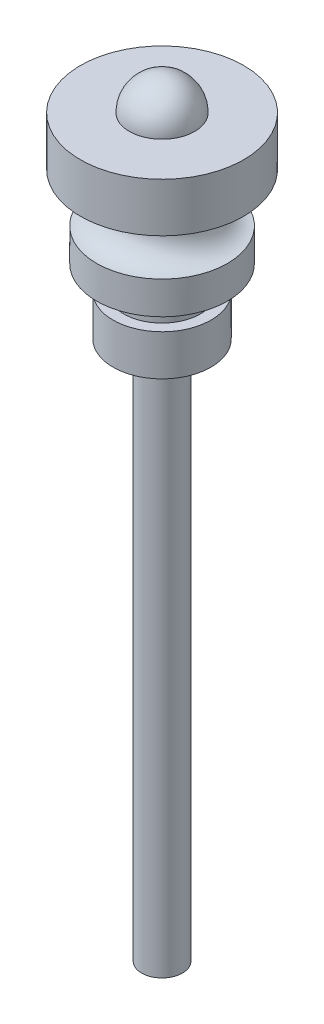
from build123d import *


with BuildPart() as part:
    # Sketch1 → Revolve1 (revolve)
    with BuildSketch(Plane.XY, mode=Mode.PRIVATE) as revolve1_sk:
        Polygon((0, 0), (10, 0), (10, -6), (8, -6), (8, -16), (4.7, -16), (4.7, -19), (6, -19), (6, -24), (2.5, -24), (2.5, -90), (0, -90), align=None)
    revolve(revolve1_sk.sketch.rotate(Axis((0, 0, 0), (0, 1, 0)), 90), axis=Axis((0, 0, 0), (0, 1, 0)))

    # Sketch2 → Cut-Revolve1 (revolve, cut)
    with BuildSketch(Plane.XY, mode=Mode.PRIVATE) as cut_revolve1_sk:
        with BuildLine():
            Line((8, -6), (17.813862568, -6))
            Line((17.813862568, -6), (17.813862568, -12))
            Line((17.813862568, -12), (8, -12))
            ThreePointArc((8, -12), (5, -9), (8, -6))
        make_face()
    revolve(cut_revolve1_sk.sketch.rotate(Axis((0, 5.105729486, 0), (0, -1, 0)), 270), axis=Axis((0, 5.105729486, 0), (0, -1, 0)), mode=Mode.SUBTRACT)

    # Sketch4 → Revolve3 (revolve)
    with BuildSketch(Plane.XY, mode=Mode.PRIVATE) as revolve3_sk:
        with BuildLine():
            Line((0, 4), (0, 0))
            Line((0, 0), (4, 0))
            ThreePointArc((4, 0), (2.828427125, 2.828427125), (0, 4))
        make_face()
    revolve(revolve3_sk.sketch.rotate(Axis((0, 4, 0), (0, -1, 0)), 90), axis=Axis((0, 4, 0), (0, -1, 0)))


solid = part.part
